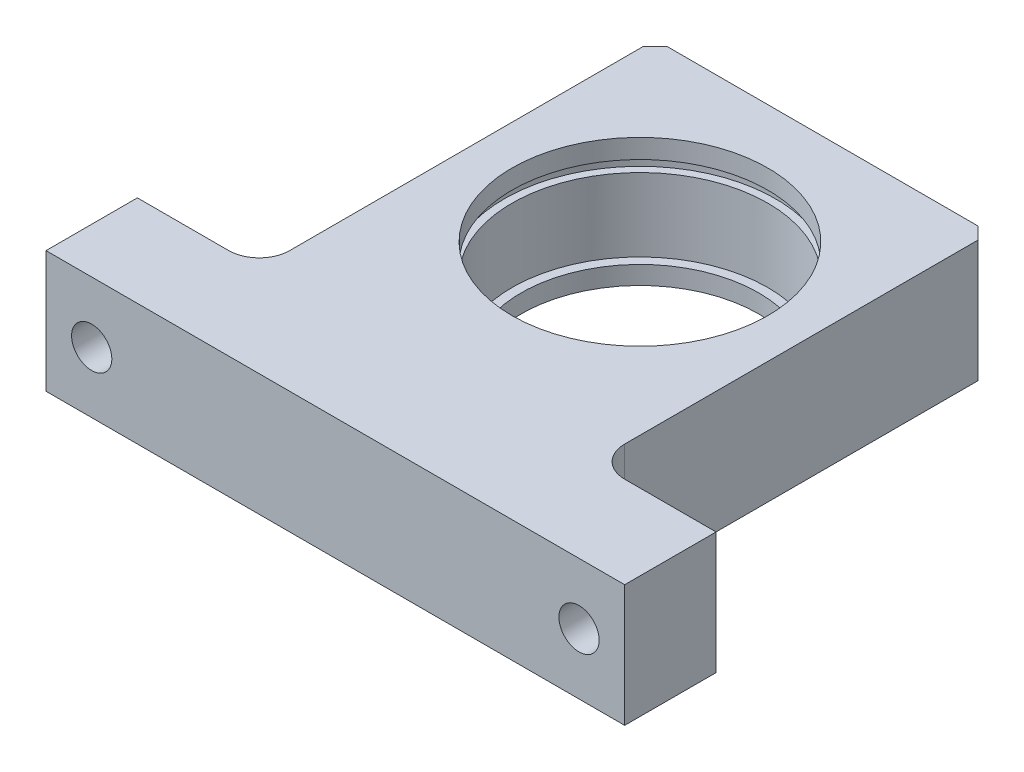
from build123d import *

# Parameters (mm, degrees)
SKETCH_1_R          = 21
EXTRUDE_1_DEPTH     = 20
CHAMFER_1_SIZE      = 2
FILLET_1_R          = 5
SKETCH_2_R          = 21
SKETCH_2_R_2        = 19.5
EXTRUDE_2_DEPTH     = 3
HOLE_WIZARD_M6_1_D  = 6.6
SKETCH_9_R          = 22.25
SKETCH_9_R_2        = 21
CUT_EXTRUDE_1_DEPTH = 1.85


with BuildPart() as part:
    # 草图1 → 凸台-拉伸1 (new body)
    with BuildSketch(Plane(origin=(0, 0, 0), x_dir=(1, 0, 0), z_dir=(0, 1, 0))):
        Polygon((-47.5, 0), (47.5, 0), (47.5, 15), (27.5, 15), (27.5, 80), (-27.5, 80), (-27.5, 15), (-47.5, 15), align=None)
        with Locations(Location((0, 50, 0), (0, 0, 270))):
            Circle(SKETCH_1_R, mode=Mode.SUBTRACT)
    extrude(amount=EXTRUDE_1_DEPTH)

    # 倒角1
    chamfer_1_edges = [part.edges().sort_by_distance(p)[0] for p in [
        (-27.5, 10, -80),
        (27.5, 10, -80),
    ]]
    chamfer(chamfer_1_edges, length=CHAMFER_1_SIZE)

    # 圆角1
    fillet_1_edges = [part.edges().sort_by_distance(p)[0] for p in [
        (-27.5, 10, -15),
        (27.5, 10, -15),
    ]]
    fillet(fillet_1_edges, radius=FILLET_1_R)

    # 草图2 → 凸台-拉伸2 (add)
    with BuildSketch(Plane.XZ):
        with Locations(Location((0, -50, 0), (0, 0, 270))):
            Circle(SKETCH_2_R)
        with Locations(Location((0, -50, 0), (0, 0, 270))):
            Circle(SKETCH_2_R_2, mode=Mode.SUBTRACT)
    extrude(amount=-EXTRUDE_2_DEPTH)

    # M6 间隙孔1 (through all)
    with Locations(Plane(origin=(0, 0, -15), x_dir=(-1, 0, 0), z_dir=(0, 0, -1))):
        with Locations((-40, 10), (40, 10)):
            Hole(HOLE_WIZARD_M6_1_D / 2)

    # 草图9 → 切除-拉伸1 (cut)
    with BuildSketch(Plane(origin=(0, 15, 0), x_dir=(1, 0, 0), z_dir=(0, 1, 0))):
        with Locations(Location((0, 50, 0), (0, 0, 270))):
            Circle(SKETCH_9_R)
        with Locations(Location((0, 50, 0), (0, 0, 90))):
            Circle(SKETCH_9_R_2, mode=Mode.SUBTRACT)
    extrude(amount=CUT_EXTRUDE_1_DEPTH, mode=Mode.SUBTRACT)


solid = part.part
